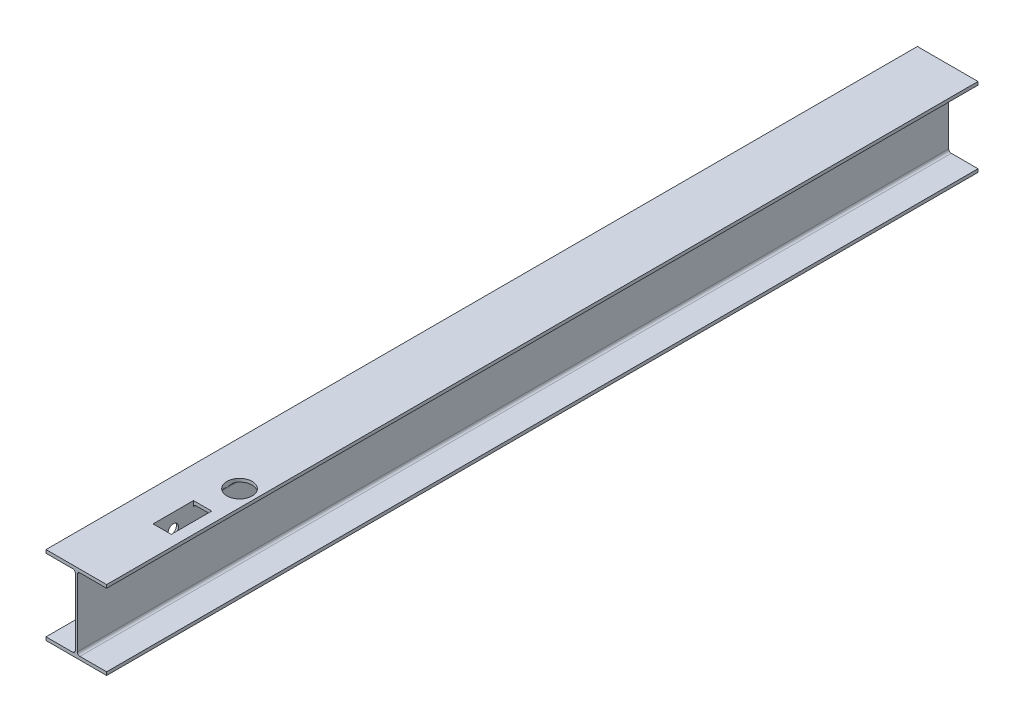
from build123d import *

# Parameters (mm, degrees)
BOSS_EXTRUDE1_DEPTH = 4313
CUT_EXTRUDE1_REACH  = 4342.976
SKETCH2_R           = 62.5
SKETCH2_W           = 90
SKETCH2_H           = 200
CUT_EXTRUDE2_REACH  = 4335.37
SKETCH3_R           = 25.5


with BuildPart() as part:
    # Sketch1 → Boss-Extrude1 (new body)
    with BuildSketch(Plane.XY):
        with BuildLine():
            Line((0, 0), (300, 0))
            Line((300, 0), (300, 16))
            Line((300, 16), (168, 16))
            ThreePointArc((168, 16), (158.807611845, 19.807611845), (155, 29))
            Line((155, 29), (155, 361))
            ThreePointArc((155, 361), (158.807611845, 370.192388155), (168, 374))
            Line((168, 374), (300, 374))
            Line((300, 374), (300, 390))
            Line((300, 390), (0, 390))
            Line((0, 390), (0, 374))
            Line((0, 374), (132, 374))
            ThreePointArc((132, 374), (141.192388155, 370.192388155), (145, 361))
            Line((145, 361), (145, 29))
            ThreePointArc((145, 29), (141.192388155, 19.807611845), (132, 16))
            Line((132, 16), (0, 16))
            Line((0, 16), (0, 0))
        make_face()
    extrude(amount=BOSS_EXTRUDE1_DEPTH)

    # Sketch2 → Cut-Extrude1 (cut, up to next)
    with BuildSketch(Plane(origin=(0, 390, 0), x_dir=(1, 0, 0), z_dir=(0, 1, 0)), mode=Mode.PRIVATE) as cut_extrude1_sk1:
        with Locations(Location((218, -3573, 0), (0, 0, 270))):
            Circle(SKETCH2_R)
    cut_extrude1_tool1 = extrude(cut_extrude1_sk1.sketch, amount=-CUT_EXTRUDE1_REACH, mode=Mode.PRIVATE) & part.part
    # Sketch2 → Cut-Extrude1 (cut, up to next)
    with BuildSketch(Plane(origin=(0, 390, 0), x_dir=(1, 0, 0), z_dir=(0, 1, 0)), mode=Mode.PRIVATE) as cut_extrude1_sk2:
        with Locations((200, -3838)):
            Rectangle(SKETCH2_W, SKETCH2_H)
    cut_extrude1_tool2 = extrude(cut_extrude1_sk2.sketch, amount=-CUT_EXTRUDE1_REACH, mode=Mode.PRIVATE) & part.part
    add(cut_extrude1_tool1.solids().sort_by_distance((218, 390, 3573))[0], mode=Mode.SUBTRACT)
    add(cut_extrude1_tool2.solids().sort_by_distance((200, 390, 3838))[0], mode=Mode.SUBTRACT)

    # Sketch3 → Cut-Extrude2 (cut, up to next)
    with BuildSketch(Plane(origin=(155, 0, 0), x_dir=(0, 0, -1), z_dir=(1, 0, 0)), mode=Mode.PRIVATE) as cut_extrude2_sk1:
        with Locations((-3838, 315)):
            Circle(SKETCH3_R)
    cut_extrude2_tool1 = extrude(cut_extrude2_sk1.sketch, amount=-CUT_EXTRUDE2_REACH, mode=Mode.PRIVATE) & part.part
    add(cut_extrude2_tool1.solids().sort_by_distance((155, 315, 3838))[0], mode=Mode.SUBTRACT)


solid = part.part
